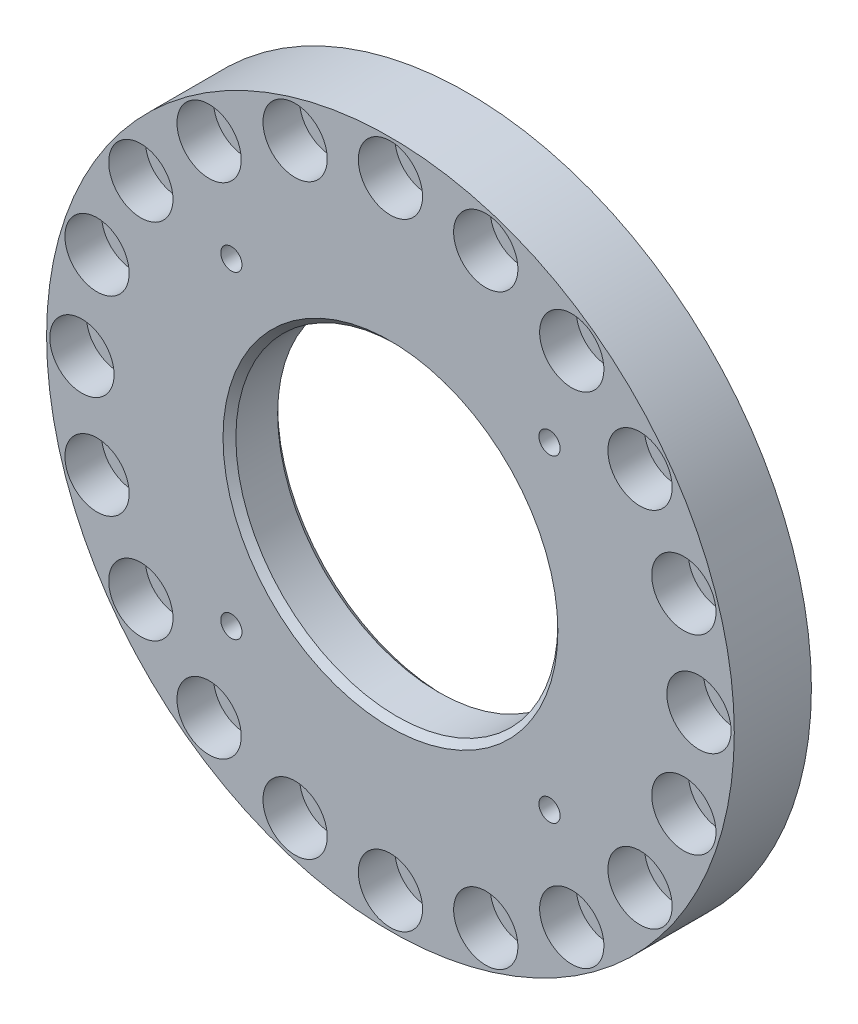
SolidWorks part; units mm, degrees
material "AL6061"
ref_plane "前视基准面" through (0, 0, 0) normal (0, 0, 1) x (1, 0, 0)
ref_plane "上视基准面" through (0, 0, 0) normal (0, 1, 0) x (1, 0, 0)
ref_plane "右视基准面" through (0, 0, 0) normal (1, 0, 0) x (0, 0, -1)
sketch "草图1" plane through (0, 0, 0) normal (0, 0, 1) x (1, 0, 0)
  circle A0 centre (0, 0) radius 25.05
  circle A1 centre (0, 0) radius 53.5
  dimension "D1" = 50.1
  dimension "D2" = 107
extrude "凸台-拉伸1" add sketch "草图1" along normal mid plane 12
hole_wizard "打孔尺寸(%根据)内六角圆柱头螺钉的类型1" positions "草图2" profile "草图3" counterbore size "M5" standard "GB" end condition through all
sketch "草图2" plane through (0, 0, 6) normal (0, 0, 1) x (1, 0, 0)
  line L0 (0, 55.0105) -> (0, -35.9518) construction
  circle A0 centre (0, 0) radius 48 construction
  point P0 (0, 48)
  dimension "D1" = 96
sketch "草图3" plane through (0, 48, 6) normal (1, 0, 0) x (0, -1, 0)
  line L0 (0, 0) -> (0, 12)
  line L1 (0, 12) -> (2.75, 12)
  line L3 (2.75, 12) -> (2.75, 5.7)
  line L4 (2.75, 5.7) -> (5, 5.7)
  line L5 (5, 5.7) -> (5, 0)
  line L7 (5, 0) -> (0, 0)
  line L11 (0, -6.35) -> (0, 107.95) construction
  dimension "通孔孔直径" = 5.5
  dimension "通孔孔深度" = 12
  dimension "柱形沉头孔直径" = 10
  dimension "柱形沉头孔深度" = 5.7
sketch "草图6" plane through (0, 0, -6) normal (0, 0, -1) x (-1, 0, 0)
  circle A0 centre (0, 0) radius 33.55
  dimension "D1" = 67.1
extrude "切除-拉伸1" cut sketch "草图6" against normal blind 3.5
chamfer "倒角1" distance 1 angle 45 3 edges at (25.05, 0, 6) (-25.05, 0, -2.5) (-33.55, 0, -6)
hole_wizard "M4 螺纹孔1" positions "草图4" profile "草图5" tap size "M4" standard "GB" end condition through all
sketch "草图4" plane through (0, 0, 6) normal (0, 0, 1) x (1, 0, 0)
  line L0 (-56.5699, 0) -> (60.5549, 0) construction
  line L2 (0, 57.956) -> (0, -57.7827) construction
  line L4 (-24.7487, 24.7487) -> (24.7487, 24.7487) construction
  line L5 (-24.7487, 24.7487) -> (-24.7487, -24.7487) construction
  line L6 (-24.7487, -24.7487) -> (24.7487, -24.7487) construction
  line L7 (24.7487, 24.7487) -> (24.7487, -24.7487) construction
  line L8 (0, 0) -> (35.0278, 35.0278) construction
  circle A0 centre (0, 0) radius 35 construction
  point P2 (24.7487, 24.7487)
  dimension "D1" = 70
  dimension "D2" = 45
sketch "草图5" plane through (24.7487, 24.7487, 6) normal (1, 0, 0) x (0, -1, 0)
  line L0 (0, 0) -> (0, 12)
  line L1 (0, 12) -> (1.65, 12)
  line L2 (1.65, 12) -> (1.65, 0)
  line L5 (1.65, 0) -> (0, 0)
  line L11 (0, -6.35) -> (0, 107.95) construction
  dimension "通孔螺纹孔钻头直径" = 3.3
  dimension "通孔螺纹孔钻头深度" = 12
cosmetic thread "孔螺蚊线1" parameters "D2"=4
pattern_circular "阵列(圆周)1" count 20 over 360 about axis through (0, 0, 0) along (0, 0, 1) of "打孔尺寸(%根据)内六角圆柱头螺钉的类型1"
pattern_circular "阵列(圆周)2" count 4 over 360 about axis through (0, 0, 0) along (0, 0, 1) of "M4 螺纹孔1"
